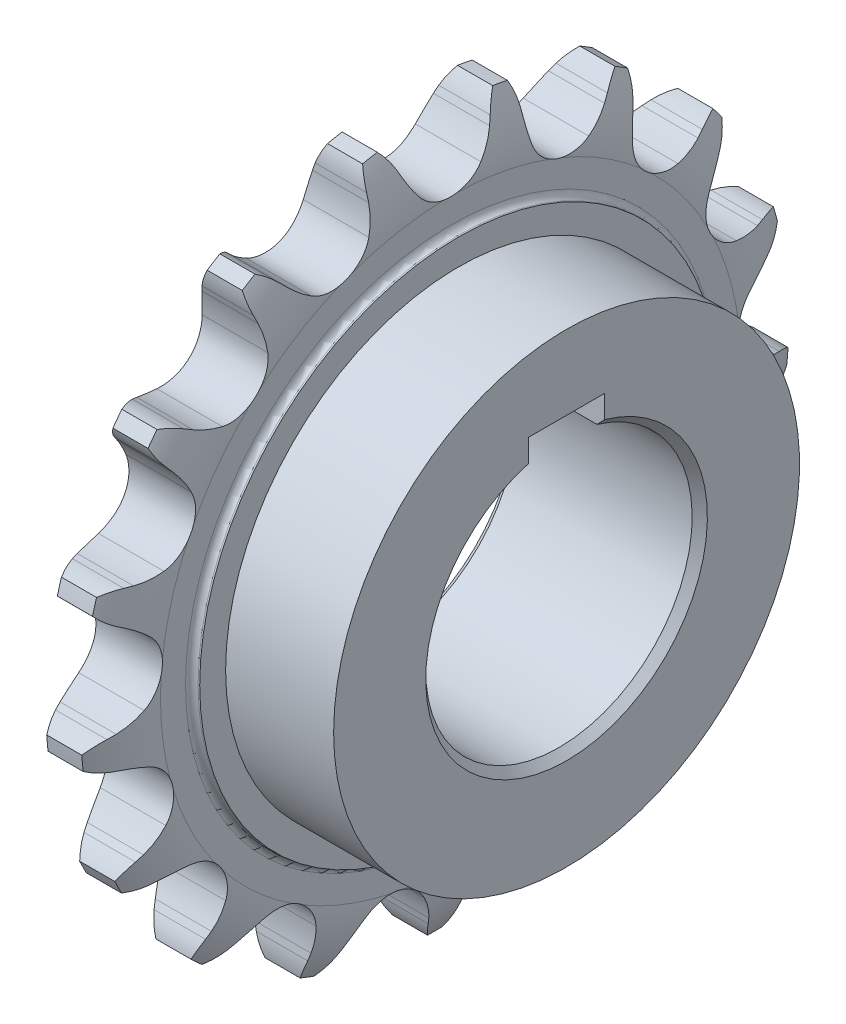
from build123d import *

# Parameters (mm, degrees)
CUT_EXTRUDE_1_DEPTH      = 5.405906443
PATTERN_CIRCULAR_1_COUNT = 17
SKETCH_3_W               = 14.188187114
SKETCH_3_H               = 13.097281179
SKETCH_4_W               = 10
SKETCH_4_H               = 4.029490121
CUT_EXTRUDE_2_DEPTH      = 71.274580331
CHAMFER_1_SIZE           = 1
CHAMFER_2_SIZE           = 1


with BuildPart() as part:
    # 草图1 → 旋转1 (revolve)
    with BuildSketch(Plane.XY, mode=Mode.PRIVATE) as revolve_1_sk:
        with BuildLine():
            Line((-5.405906443, 17.5), (-5.405906443, 34))
            Line((-5.405906443, 34), (-5.198925154, 34))
            ThreePointArc((-5.198925154, 34), (-4.613493663, 34.242493663), (-4.371, 34.827925154))
            Line((-4.371, 34.827925154), (-4.371, 38.117392267))
            ThreePointArc((-4.371, 38.117392267), (-3.919878552, 42.451674331), (-2.30725, 46.5))
            Line((-2.30725, 46.5), (2.30725, 46.5))
            ThreePointArc((2.30725, 46.5), (3.919878552, 42.451674331), (4.371, 38.117392267))
            Line((4.371, 38.117392267), (4.371, 34.827925154))
            ThreePointArc((4.371, 34.827925154), (4.613493663, 34.242493663), (5.198925154, 34))
            Line((5.198925154, 34), (5.405906443, 34))
            Line((5.405906443, 34), (5.405906443, 17.5))
            Line((5.405906443, 17.5), (-5.405906443, 17.5))
        make_face()
    revolve(revolve_1_sk.sketch.rotate(Axis((-7.9375, 0, 0), (1, 0, 0)), 90), axis=Axis((-7.9375, 0, 0), (1, 0, 0)))

    # 草图2 → 切除-拉伸1 (cut, symmetric)
    with BuildSketch(Plane(origin=(0, 0, 0), x_dir=(0, 0, -1), z_dir=(1, 0, 0))):
        with BuildLine():
            Line((5.793131969, 42.895011616), (6.18114945, 43.773787436))
            ThreePointArc((6.18114945, 43.773787436), (6.790313357, 44.8857779), (7.579548398, 45.878104212))
            ThreePointArc((7.579548398, 45.878104212), (0, 46.5), (-7.579548398, 45.878104212))
            ThreePointArc((-7.579548398, 45.878104212), (-6.790313357, 44.8857779), (-6.18114945, 43.773787436))
            Line((-6.18114945, 43.773787436), (-5.793131969, 42.895011616))
            ThreePointArc((-5.793131969, 42.895011616), (-5.006529608, 41.38396254), (-4.033010117, 39.986009613))
            ThreePointArc((-4.033010117, 39.986009613), (0, 38.041992267), (4.033010117, 39.986009613))
            ThreePointArc((4.033010117, 39.986009613), (5.006529608, 41.38396254), (5.793131969, 42.895011616))
        make_face()
    cut_extrude_1 = extrude(amount=CUT_EXTRUDE_1_DEPTH, both=True, mode=Mode.SUBTRACT)

    # 阵列(圆周)1: 切除-拉伸1 ×17 about axis
    pattern_circular_1_axis = Axis((0, 0, 0), (1, 0, 0))
    for i in range(1, PATTERN_CIRCULAR_1_COUNT):
        add(cut_extrude_1.rotate(pattern_circular_1_axis, i * 360 / PATTERN_CIRCULAR_1_COUNT), mode=Mode.SUBTRACT)

    # 草图3 → 旋转2 (revolve)
    with BuildSketch(Plane.XY, mode=Mode.PRIVATE) as revolve_2_sk:
        with Locations((12.5, 24.04864059)):
            Rectangle(SKETCH_3_W, SKETCH_3_H)
    revolve(revolve_2_sk.sketch.rotate(Axis((0, 0, 0), (1, 0, 0)), 90), axis=Axis((0, 0, 0), (1, 0, 0)))

    # 草图4 → 切除-拉伸2 (cut, through all)
    with BuildSketch(Plane.ZY.offset(5.405906443)):
        with Locations((0, 18.785254892)):
            Rectangle(SKETCH_4_W, SKETCH_4_H)
    extrude(amount=-CUT_EXTRUDE_2_DEPTH, mode=Mode.SUBTRACT)

    # 倒角1
    chamfer_1_edges = [part.edges().sort_by_distance(p)[0] for p in [
        (-5.405906443, -17.5, 0),
    ]]
    chamfer(chamfer_1_edges, length=CHAMFER_1_SIZE)

    # 倒角2
    chamfer_2_edges = [part.edges().sort_by_distance(p)[0] for p in [
        (19.594093557, -17.5, 0),
    ]]
    chamfer(chamfer_2_edges, length=CHAMFER_2_SIZE)


solid = part.part
